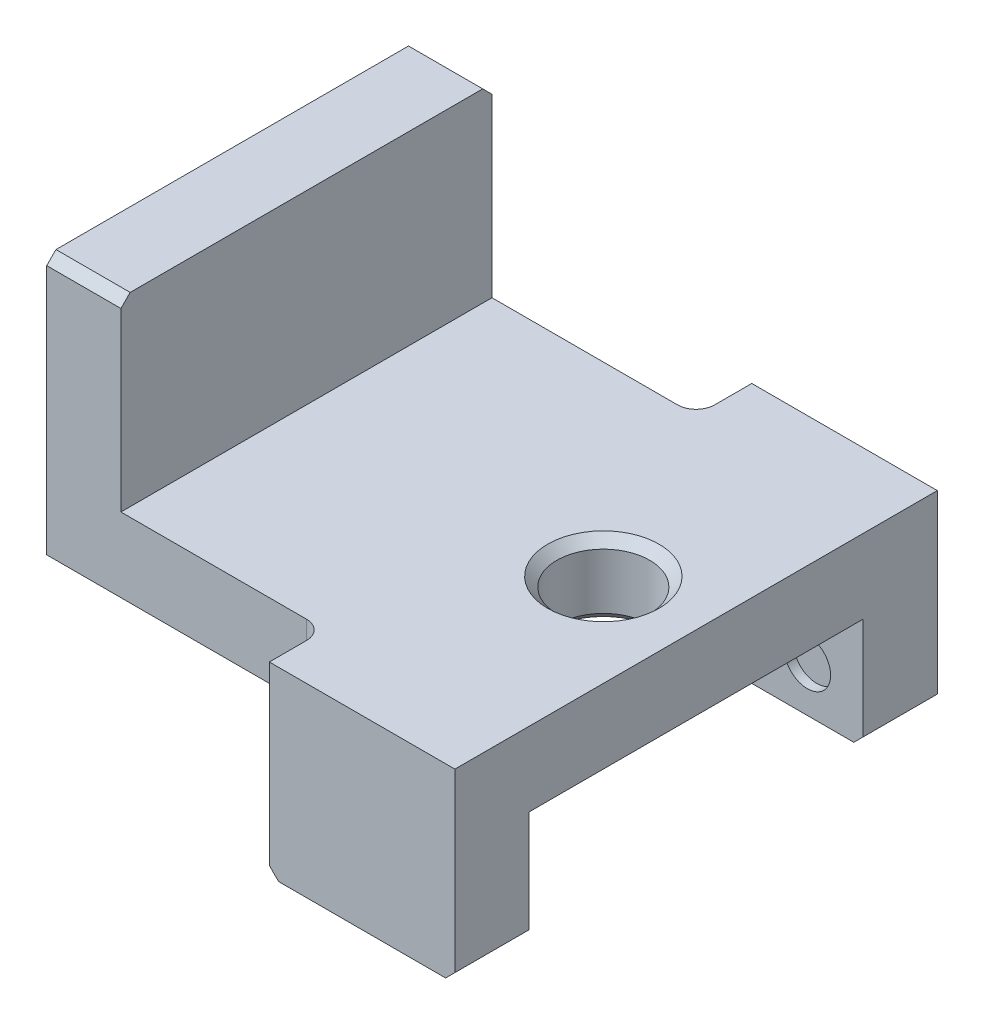
from build123d import *

# Parameters (mm, degrees)
SKETCH1_W           = 50
SKETCH1_H           = 40
BOSS_EXTRUDE1_DEPTH = 8
SKETCH3_W           = 20
SKETCH3_H           = 52
BOSS_EXTRUDE2_DEPTH = 8
SKETCH2_R           = 5
CUT_EXTRUDE1_DEPTH  = 69.410525506
CHAMFER2_SIZE       = 1
SKETCH4_W           = 20
SKETCH4_H           = 8
BOSS_EXTRUDE3_DEPTH = 12
CHAMFER4_SIZE       = 1
FILLET1_R           = 2
SKETCH5_W           = 8
SKETCH5_H           = 40
BOSS_EXTRUDE4_DEPTH = 20
CHAMFER5_SIZE       = 1
SKETCH6_R           = 2.5
CUT_EXTRUDE2_DEPTH  = 1
CUT_EXTRUDE3_START  = -1
SKETCH7_R           = 2.5
CUT_EXTRUDE3_DEPTH  = 1


with BuildPart() as part:
    # Sketch1 → Boss-Extrude1 (new body)
    with BuildSketch(Plane(origin=(0, 0, 0), x_dir=(1, 0, 0), z_dir=(0, 1, 0))):
        with Locations((25, -20)):
            Rectangle(SKETCH1_W, SKETCH1_H)
    extrude(amount=BOSS_EXTRUDE1_DEPTH)

    # Sketch3 → Boss-Extrude2 (add)
    with BuildSketch(Plane(origin=(0, 8, 0), x_dir=(1, 0, 0), z_dir=(0, 1, 0))):
        with Locations((40, -20)):
            Rectangle(SKETCH3_W, SKETCH3_H)
    extrude(amount=-BOSS_EXTRUDE2_DEPTH)

    # Sketch2 → Cut-Extrude1 (cut, through all)
    with BuildSketch(Plane.XZ):
        with Locations(Location((40, 20, 0), (0, 0, 270))):
            Circle(SKETCH2_R)
    extrude(amount=-CUT_EXTRUDE1_DEPTH, mode=Mode.SUBTRACT)

    # Chamfer2
    chamfer2_edges = [part.edges().sort_by_distance(p)[0] for p in [
        (40, 8, 25),
        (40, 0, 25),
    ]]
    chamfer(chamfer2_edges, length=CHAMFER2_SIZE)

    # Sketch4 → Boss-Extrude3 (add)
    with BuildSketch(Plane(origin=(0, 0, 0), x_dir=(1, 0, 0), z_dir=(0, 1, 0))):
        with Locations((40, -42)):
            Rectangle(SKETCH4_W, SKETCH4_H)
        with Locations((40, 2)):
            Rectangle(SKETCH4_W, SKETCH4_H)
    extrude(amount=-BOSS_EXTRUDE3_DEPTH)

    # Chamfer4
    chamfer4_edges = [part.edges().sort_by_distance(p)[0] for p in [
        (30, -12, 42),
        (50, -12, 42),
        (30, -12, -2),
        (50, -12, -2),
    ]]
    chamfer(chamfer4_edges, length=CHAMFER4_SIZE)

    # Fillet1
    fillet1_edges = [part.edges().sort_by_distance(p)[0] for p in [
        (30, 4, 40),
        (30, 4, 0),
    ]]
    fillet(fillet1_edges, radius=FILLET1_R)

    # Sketch5 → Boss-Extrude4 (add)
    with BuildSketch(Plane(origin=(0, 8, 0), x_dir=(1, 0, 0), z_dir=(0, 1, 0))):
        with Locations((4, -20)):
            Rectangle(SKETCH5_W, SKETCH5_H)
    extrude(amount=BOSS_EXTRUDE4_DEPTH)

    # Chamfer5
    chamfer5_edges = [part.edges().sort_by_distance(p)[0] for p in [
        (4, 28, 40),
        (4, 28, 0),
    ]]
    chamfer(chamfer5_edges, length=CHAMFER5_SIZE)

    # Sketch6 → Cut-Extrude2 (cut)
    with BuildSketch(Plane.XY.offset(2)):
        with Locations((44, -7)):
            Circle(SKETCH6_R)
        with Locations((36, -7)):
            Circle(SKETCH6_R)
    extrude(amount=-CUT_EXTRUDE2_DEPTH, mode=Mode.SUBTRACT)

    # Sketch7 → Cut-Extrude3 (cut)
    with BuildSketch(Plane(origin=(0, 0, 38), x_dir=(-1, 0, 0), z_dir=(0, 0, -1)).offset(CUT_EXTRUDE3_START)):
        with Locations(Location((-36, -7, 0), (0, 0, 180))):
            Circle(SKETCH7_R)
        with Locations(Location((-44, -7, 0), (0, 0, 180))):
            Circle(SKETCH7_R)
    extrude(amount=CUT_EXTRUDE3_DEPTH, mode=Mode.SUBTRACT)


solid = part.part
